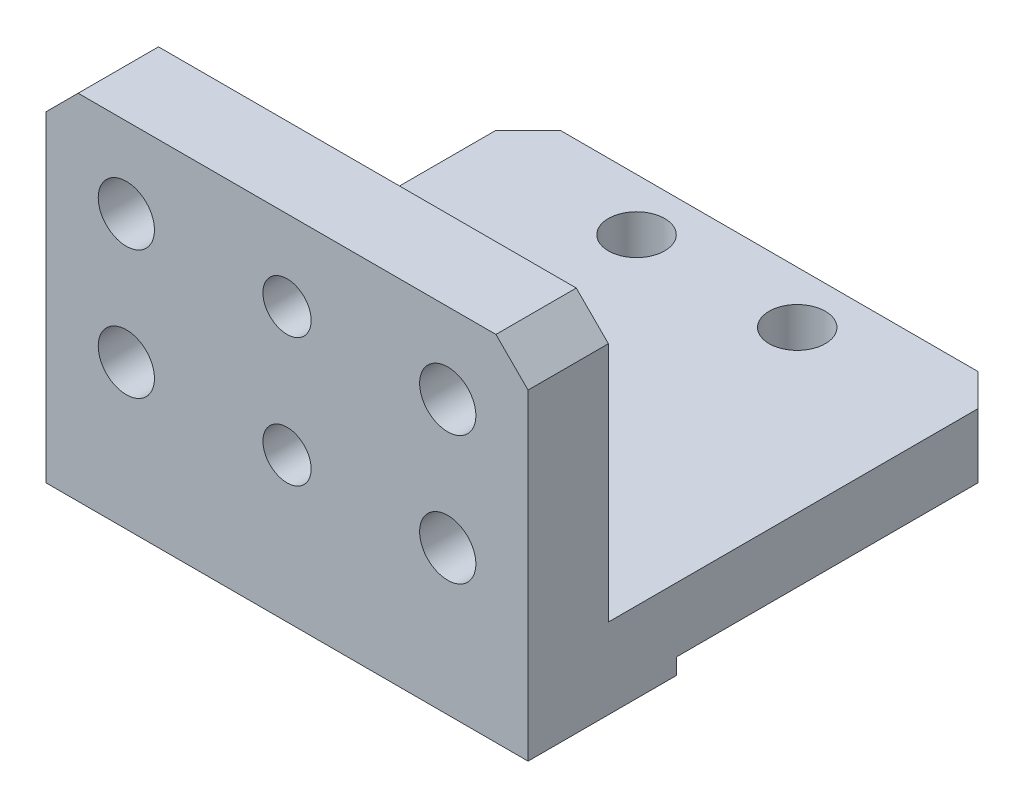
SolidWorks part; units mm, degrees
material "A6061 T6"
ref_plane "前视基准面" through (0, 0, 0) normal (0, 0, 1) x (1, 0, 0)
ref_plane "上视基准面" through (0, 0, 0) normal (0, 1, 0) x (1, 0, 0)
ref_plane "右视基准面" through (0, 0, 0) normal (1, 0, 0) x (0, 0, -1)
sketch "草图1" plane through (0, 0, 0) normal (0, 1, 0) x (1, 0, 0)
  line L1 (-15, 15) -> (15, 15)
  line L2 (-15, 15) -> (-15, -15)
  line L3 (-15, -15) -> (15, -15)
  line L4 (15, 15) -> (15, -15)
  line L5 (-15, 15) -> (15, -15) construction
  line L6 (-15, -15) -> (15, 15) construction
  point P0 (0, 0)
  dimension "D1" = 30
  dimension "D2" = 30
extrude "凸台-拉伸1" add sketch "草图1" along normal blind 5
sketch "草图2" plane through (0, 5, 0) normal (0, 1, 0) x (1, 0, 0)
  line L0 (15, -15) -> (15, 15) construction
  line L1 (-15, -15) -> (15, -15)
  line L2 (-15, -15) -> (-15, -10)
  line L3 (-15, -10) -> (15, -10)
  line L4 (15, -15) -> (15, -10)
  dimension "D1" = 5
extrude "凸台-拉伸2" add sketch "草图2" along normal blind 17
hole_wizard "Ø3.5 (3.5) 直径孔1" positions "草图3" profile "草图4" hole size "Ø3.5" standard "GB"
sketch "草图3" plane through (0, 5, 0) normal (0, 1, 0) x (1, 0, 0)
  point P0 (-5, 11.75)
  point P3 (5, 11.75)
  point P6 (5, -3.25)
  point P9 (-5, -3.25)
sketch "草图4" plane through (-5, 5, -11.75) normal (1, 0, 0) x (0, 0, 1)
  line L0 (0, 0) -> (0, 13.4515)
  line L1 (0, 13.4515) -> (1.75, 12.4)
  line L2 (1.75, 12.4) -> (1.75, 0)
  line L5 (1.75, 0) -> (0, 0)
  line L10 (0, 13.4515) -> (-1.75, 12.4) construction
  line L11 (0, -6.35) -> (0, 107.95) construction
  dimension "孔直径" = 3.5
  dimension "孔深度" = 12.4
  dimension "导头角度" = 118
sketch "草图5" plane through (-15, 0, 0) normal (-1, 0, 0) x (0, 0, 1)
  line L1 (-15, 0) -> (5.75, 0)
  line L2 (-15, 0) -> (-15, 1)
  line L3 (-15, 1) -> (5.75, 1)
  line L4 (5.75, 0) -> (5.75, 1)
  dimension "D1" = 20.75
  dimension "D2" = 1
extrude "切除-拉伸1" cut sketch "草图5" against normal through all
chamfer "倒角1" distance 2 angle 45 4 edges at (-15, 3, -15) (15, 3, -15) (-15, 22, 12.5) (15, 22, 12.5)
hole_wizard "Ø3.5 (3.5) 直径孔2" positions "草图6" profile "草图7" hole size "Ø3.5" standard "GB"
sketch "草图6" plane through (0, 0, 10) normal (0, 0, -1) x (-1, 0, 0)
  line L0 (-13, 22) -> (13, 22) construction
  line L1 (15, 20) -> (15, 5) construction
  line L2 (-15, 20) -> (-15, 5) construction
  point P0 (-10, 17)
  point P2 (10, 17)
  point P4 (-10, 9)
  point P6 (10, 9)
  dimension "D1" = 5
  dimension "D2" = 8
  dimension "D3" = 5
  dimension "D4" = 5
sketch "草图7" plane through (10, 17, 10) normal (1, 0, 0) x (0, 1, 0)
  line L0 (0, 0) -> (0, 13.4515)
  line L1 (0, 13.4515) -> (1.75, 12.4)
  line L2 (1.75, 12.4) -> (1.75, 0)
  line L5 (1.75, 0) -> (0, 0)
  line L10 (0, 13.4515) -> (-1.75, 12.4) construction
  line L11 (0, -6.35) -> (0, 107.95) construction
  dimension "孔直径" = 3.5
  dimension "孔深度" = 12.4
  dimension "导头角度" = 118
hole_wizard "大小mm 暗销孔1" positions "草图8" profile "草图9" hole size "Ø3.0" standard "GB"
sketch "草图8" plane through (0, 0, 10) normal (0, 0, -1) x (-1, 0, 0)
  line L0 (-13, 22) -> (13, 22) construction
  line L1 (-15, 20) -> (-15, 5) construction
  point P0 (0, 17)
  point P2 (0, 9)
  dimension "D1" = 5
  dimension "D2" = 8
  dimension "D3" = 15
sketch "草图9" plane through (0, 17, 10) normal (1, 0, 0) x (0, 1, 0)
  line L0 (0, 0) -> (0, 13.3013)
  line L1 (0, 13.3013) -> (1.5, 12.4)
  line L2 (1.5, 12.4) -> (1.5, 0)
  line L5 (1.5, 0) -> (0, 0)
  line L10 (0, 13.3013) -> (-1.5, 12.4) construction
  line L11 (0, -6.35) -> (0, 107.95) construction
  dimension "孔直径" = 3
  dimension "孔深度" = 12.4
  dimension "导头角度" = 118
